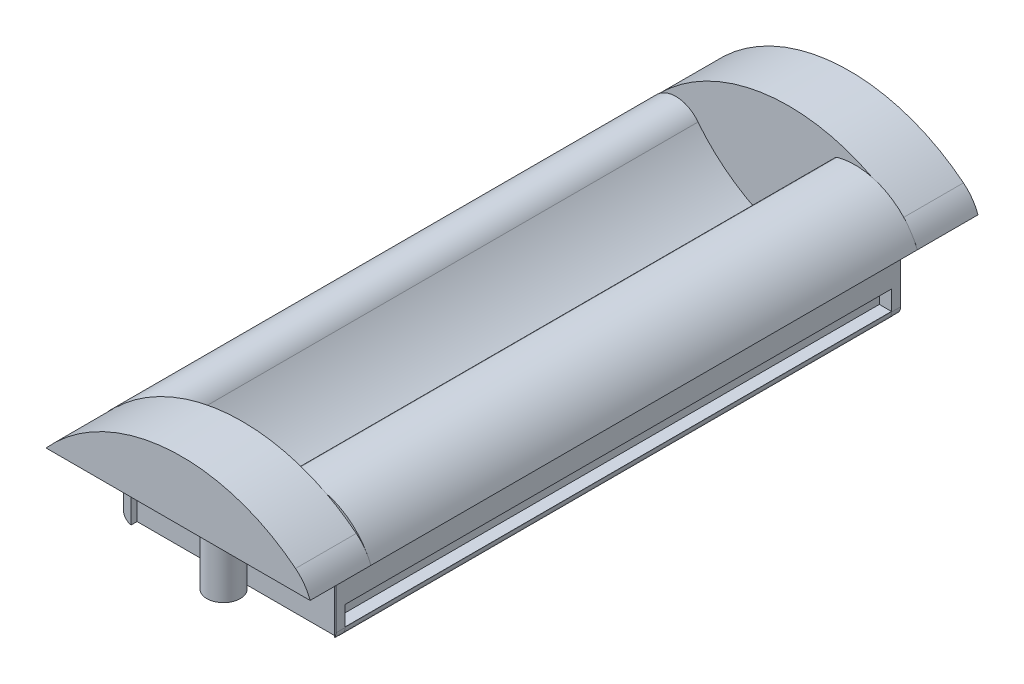
from build123d import *

# Parameters (mm, degrees)
EXTRUDE_1_DEPTH      = 45
EXTRUDE_2_DEPTH      = 10
CUT_EXTRUDE_11_DEPTH = 12.5
FILLET_1_R           = 1.5
SKETCH_4_R           = 1.7
CUT_EXTRUDE_12_DEPTH = 11.25


with BuildPart() as part:
    # 草图1 → 凸台-拉伸1 (new, symmetric)
    with BuildSketch(Plane.XY):
        with BuildLine():
            Line((-15.5, 0), (15.5, 0))
            ThreePointArc((15.5, 0), (16.560660172, 0.439339828), (17, 1.5))
            Line((17, 1.5), (17, 1.6))
            Line((17, 1.6), (15, 1.6))
            Line((15, 1.6), (15, 4.8))
            Line((15, 4.8), (17, 4.8))
            Line((17, 4.8), (17, 12.5))
            Line((17, 12.5), (21.25, 12.5))
            ThreePointArc((21.25, 12.5), (15.900063146, 18.351194202), (8.005834372, 19.085666803))
            ThreePointArc((8.005834372, 19.085666803), (7.659690231, 18.472905768), (8.269164703, 18.121007034))
            ThreePointArc((8.269164703, 18.121007034), (13.386035944, 17.124613538), (15.791887335, 12.5))
            ThreePointArc((15.791887335, 12.5), (12.736961816, 4.997664438), (5.127858316, 2.219328112))
            ThreePointArc((5.127858316, 2.219328112), (-5.972198102, 5.342922516), (-14.872141684, 12.674982166))
            ThreePointArc((-14.872141684, 12.674982166), (-18.60669741, 14.511266303), (-22.25, 12.5))
            Line((-22.25, 12.5), (-18, 12.5))
            Line((-18, 12.5), (-18, 4.8))
            Line((-18, 4.8), (-15, 4.8))
            Line((-15, 4.8), (-15, 1.6))
            Line((-15, 1.6), (-17, 1.6))
            Line((-17, 1.6), (-17, 1.5))
            ThreePointArc((-17, 1.5), (-16.560660172, 0.439339828), (-15.5, 0))
        make_face()
    extrude(amount=EXTRUDE_1_DEPTH, both=True)

    # 草图2 → 凸台-拉伸2 (add)
    with BuildSketch(Plane.XY.offset(45)):
        with BuildLine():
            Line((-22.25, 12.5), (-18, 12.5))
            Line((-18, 12.5), (-18, 1.5))
            Line((-18, 1.5), (-18, 0))
            Line((-18, 0), (-16.5, 0))
            Line((-16.5, 0), (16.5, 0))
            Line((16.5, 0), (17, 0))
            Line((17, 0), (17, 1.5))
            Line((17, 1.5), (17, 12.5))
            Line((17, 12.5), (21.25, 12.5))
            ThreePointArc((21.25, 12.5), (20.28562135, 14.348675496), (18.853738793, 15.864373227))
            ThreePointArc((18.853738793, 15.864373227), (-2.367503819, 22.360156158), (-22.25, 12.5))
        make_face()
    extrude_2 = extrude(amount=EXTRUDE_2_DEPTH)

    # 镜向1: 凸台-拉伸2 across plane
    add(extrude_2.mirror(Plane.XY))

    # 草图3 → 切除-拉伸11 (cut)
    with BuildSketch(Plane.XZ):
        with BuildLine():
            Line((1.145643924, 45.5), (16.73, 45.5))
            Line((16.73, 45.5), (16.73, 46.5))
            Line((16.73, 46.5), (18, 46.5))
            Line((18, 46.5), (18, 55))
            Line((18, 55), (-18, 55))
            Line((-18, 55), (-18, 46.5))
            Line((-18, 46.5), (-16.73, 46.5))
            Line((-16.73, 46.5), (-16.73, 45.5))
            Line((-16.73, 45.5), (-1.145643924, 45.5))
            ThreePointArc((-1.145643924, 45.5), (0, 50.75), (1.145643924, 45.5))
        make_face()
        with BuildLine():
            Line((-18, -46.5), (-18, -55))
            Line((-18, -55), (18, -55))
            Line((18, -55), (18, -46.5))
            Line((18, -46.5), (16.73, -46.5))
            Line((16.73, -46.5), (16.73, -45.5))
            Line((16.73, -45.5), (1.145643924, -45.5))
            ThreePointArc((1.145643924, -45.5), (0, -50.75), (-1.145643924, -45.5))
            Line((-1.145643924, -45.5), (-16.73, -45.5))
            Line((-16.73, -45.5), (-16.73, -46.5))
            Line((-16.73, -46.5), (-18, -46.5))
        make_face()
    extrude(amount=-CUT_EXTRUDE_11_DEPTH, mode=Mode.SUBTRACT)

    # 圆角1
    fillet_1_edges = [part.edges().sort_by_distance(p)[0] for p in [
        (-18, 0, -45.75),
        (17, 0, -45.75),
        (17, 0, 45.75),
        (-18, 0, 45.75),
    ]]
    fillet(fillet_1_edges, radius=FILLET_1_R)

    # 草图4 → 切除-拉伸12 (cut)
    with BuildSketch(Plane.XZ):
        with Locations(Location((0, 48, 0), (0, 0, 270))):
            Circle(SKETCH_4_R)
        with Locations(Location((0, -48, 0), (0, 0, 270))):
            Circle(SKETCH_4_R)
    extrude(amount=-CUT_EXTRUDE_12_DEPTH, mode=Mode.SUBTRACT)


solid = part.part
